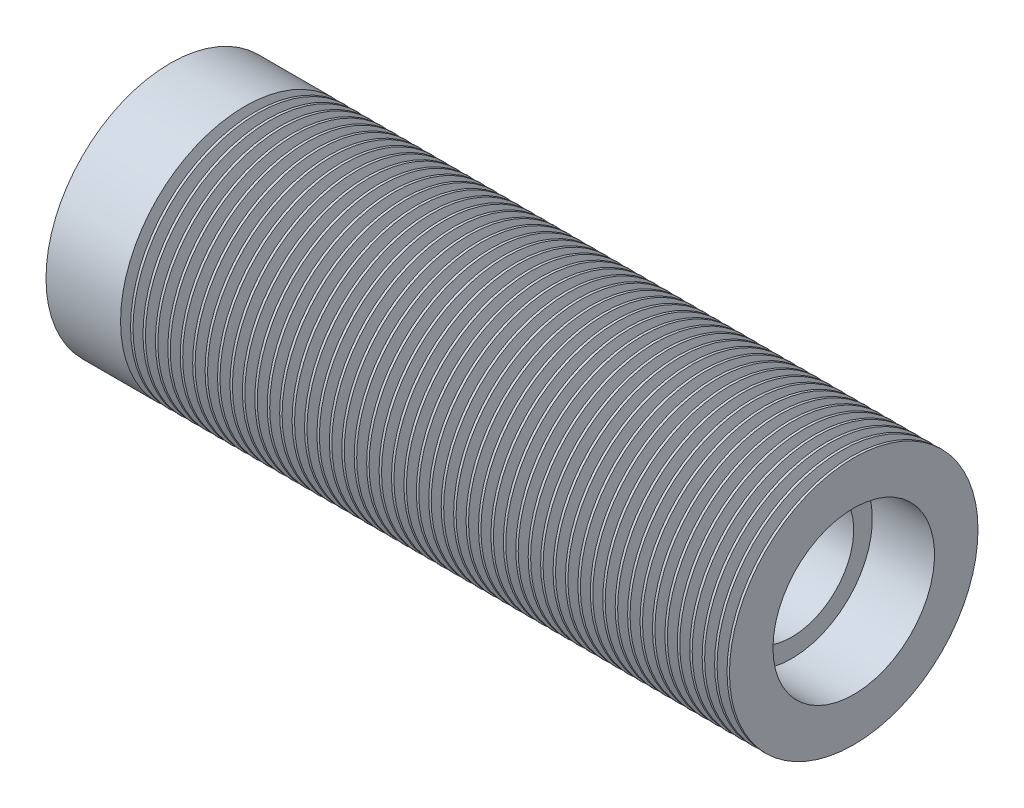
SolidWorks part; units mm, degrees
material "白色铁氟龙"
ref_plane "Front Plane" through (0, 0, 0) normal (0, 0, 1) x (1, 0, 0)
ref_plane "Top Plane" through (0, 0, 0) normal (0, 1, 0) x (1, 0, 0)
ref_plane "Right Plane" through (0, 0, 0) normal (1, 0, 0) x (0, 0, -1)
sketch "Sketch1" plane through (0, 0, 0) normal (0, 0, 1) x (1, 0, 0)
  line L0 (0, 0) -> (49.6022, 0) construction
  line L1 (0, 6.5) -> (0, 10)
  line L2 (0, 10) -> (6, 10)
  line L3 (55, 10) -> (55, 6.5)
  line L4 (55, 6.5) -> (50, 6.5)
  line L5 (50, 6.5) -> (50, 5)
  line L6 (50, 5) -> (5, 5)
  line L7 (5, 5) -> (5, 6.5)
  line L8 (5, 6.5) -> (0, 6.5)
  line L9 (6, 10) -> (6.4019, 8.5)
  line L10 (6.4019, 8.5) -> (6.8038, 10)
  line L11 (6.4019, 10) -> (6.4019, 8.5) construction
  line L12 (7, 10) -> (7.4019, 8.5)
  line L13 (7.4019, 8.5) -> (7.8038, 10)
  line L14 (7.4019, 10) -> (7.4019, 8.5) construction
  line L15 (8, 10) -> (8.4019, 8.5)
  line L16 (8.4019, 8.5) -> (8.8038, 10)
  line L17 (8.4019, 10) -> (8.4019, 8.5) construction
  line L18 (9, 10) -> (9.4019, 8.5)
  line L19 (9.4019, 8.5) -> (9.8038, 10)
  line L20 (9.4019, 10) -> (9.4019, 8.5) construction
  line L21 (10, 10) -> (10.4019, 8.5)
  line L22 (10.4019, 8.5) -> (10.8038, 10)
  line L23 (10.4019, 10) -> (10.4019, 8.5) construction
  line L24 (11, 10) -> (11.4019, 8.5)
  line L25 (11.4019, 8.5) -> (11.8038, 10)
  line L26 (11.4019, 10) -> (11.4019, 8.5) construction
  line L27 (12, 10) -> (12.4019, 8.5)
  line L28 (12.4019, 8.5) -> (12.8038, 10)
  line L29 (12.4019, 10) -> (12.4019, 8.5) construction
  line L30 (13, 10) -> (13.4019, 8.5)
  line L31 (13.4019, 8.5) -> (13.8038, 10)
  line L32 (13.4019, 10) -> (13.4019, 8.5) construction
  line L33 (14, 10) -> (14.4019, 8.5)
  line L34 (14.4019, 8.5) -> (14.8038, 10)
  line L35 (14.4019, 10) -> (14.4019, 8.5) construction
  line L36 (15, 10) -> (15.4019, 8.5)
  line L37 (15.4019, 8.5) -> (15.8038, 10)
  line L38 (15.4019, 10) -> (15.4019, 8.5) construction
  line L39 (16, 10) -> (16.4019, 8.5)
  line L40 (16.4019, 8.5) -> (16.8038, 10)
  line L41 (16.4019, 10) -> (16.4019, 8.5) construction
  line L42 (17, 10) -> (17.4019, 8.5)
  line L43 (17.4019, 8.5) -> (17.8038, 10)
  line L44 (17.4019, 10) -> (17.4019, 8.5) construction
  line L45 (18, 10) -> (18.4019, 8.5)
  line L46 (18.4019, 8.5) -> (18.8038, 10)
  line L47 (18.4019, 10) -> (18.4019, 8.5) construction
  line L48 (19, 10) -> (19.4019, 8.5)
  line L49 (19.4019, 8.5) -> (19.8038, 10)
  line L50 (19.4019, 10) -> (19.4019, 8.5) construction
  line L51 (20, 10) -> (20.4019, 8.5)
  line L52 (20.4019, 8.5) -> (20.8038, 10)
  line L53 (20.4019, 10) -> (20.4019, 8.5) construction
  line L54 (21, 10) -> (21.4019, 8.5)
  line L55 (21.4019, 8.5) -> (21.8038, 10)
  line L56 (21.4019, 10) -> (21.4019, 8.5) construction
  line L57 (22, 10) -> (22.4019, 8.5)
  line L58 (22.4019, 8.5) -> (22.8038, 10)
  line L59 (22.4019, 10) -> (22.4019, 8.5) construction
  line L60 (23, 10) -> (23.4019, 8.5)
  line L61 (23.4019, 8.5) -> (23.8038, 10)
  line L62 (23.4019, 10) -> (23.4019, 8.5) construction
  line L63 (24, 10) -> (24.4019, 8.5)
  line L64 (24.4019, 8.5) -> (24.8038, 10)
  line L65 (24.4019, 10) -> (24.4019, 8.5) construction
  line L66 (25, 10) -> (25.4019, 8.5)
  line L67 (25.4019, 8.5) -> (25.8038, 10)
  line L68 (25.4019, 10) -> (25.4019, 8.5) construction
  line L69 (26, 10) -> (26.4019, 8.5)
  line L70 (26.4019, 8.5) -> (26.8038, 10)
  line L71 (26.4019, 10) -> (26.4019, 8.5) construction
  line L72 (27, 10) -> (27.4019, 8.5)
  line L73 (27.4019, 8.5) -> (27.8038, 10)
  line L74 (27.4019, 10) -> (27.4019, 8.5) construction
  line L75 (28, 10) -> (28.4019, 8.5)
  line L76 (28.4019, 8.5) -> (28.8038, 10)
  line L77 (28.4019, 10) -> (28.4019, 8.5) construction
  line L78 (29, 10) -> (29.4019, 8.5)
  line L79 (29.4019, 8.5) -> (29.8038, 10)
  line L80 (29.4019, 10) -> (29.4019, 8.5) construction
  line L81 (30, 10) -> (30.4019, 8.5)
  line L82 (30.4019, 8.5) -> (30.8038, 10)
  line L83 (30.4019, 10) -> (30.4019, 8.5) construction
  line L84 (31, 10) -> (31.4019, 8.5)
  line L85 (31.4019, 8.5) -> (31.8038, 10)
  line L86 (31.4019, 10) -> (31.4019, 8.5) construction
  line L87 (32, 10) -> (32.4019, 8.5)
  line L88 (32.4019, 8.5) -> (32.8038, 10)
  line L89 (32.4019, 10) -> (32.4019, 8.5) construction
  line L90 (33, 10) -> (33.4019, 8.5)
  line L91 (33.4019, 8.5) -> (33.8038, 10)
  line L92 (33.4019, 10) -> (33.4019, 8.5) construction
  line L93 (34, 10) -> (34.4019, 8.5)
  line L94 (34.4019, 8.5) -> (34.8038, 10)
  line L95 (34.4019, 10) -> (34.4019, 8.5) construction
  line L96 (35, 10) -> (35.4019, 8.5)
  line L97 (35.4019, 8.5) -> (35.8038, 10)
  line L98 (35.4019, 10) -> (35.4019, 8.5) construction
  line L99 (36, 10) -> (36.4019, 8.5)
  line L100 (36.4019, 8.5) -> (36.8038, 10)
  line L101 (36.4019, 10) -> (36.4019, 8.5) construction
  line L102 (37, 10) -> (37.4019, 8.5)
  line L103 (37.4019, 8.5) -> (37.8038, 10)
  line L104 (37.4019, 10) -> (37.4019, 8.5) construction
  line L105 (38, 10) -> (38.4019, 8.5)
  line L106 (38.4019, 8.5) -> (38.8038, 10)
  line L107 (38.4019, 10) -> (38.4019, 8.5) construction
  line L108 (39, 10) -> (39.4019, 8.5)
  line L109 (39.4019, 8.5) -> (39.8038, 10)
  line L110 (39.4019, 10) -> (39.4019, 8.5) construction
  line L111 (40, 10) -> (40.4019, 8.5)
  line L112 (40.4019, 8.5) -> (40.8038, 10)
  line L113 (40.4019, 10) -> (40.4019, 8.5) construction
  line L114 (41, 10) -> (41.4019, 8.5)
  line L115 (41.4019, 8.5) -> (41.8038, 10)
  line L116 (41.4019, 10) -> (41.4019, 8.5) construction
  line L117 (42, 10) -> (42.4019, 8.5)
  line L118 (42.4019, 8.5) -> (42.8038, 10)
  line L119 (42.4019, 10) -> (42.4019, 8.5) construction
  line L120 (43, 10) -> (43.4019, 8.5)
  line L121 (43.4019, 8.5) -> (43.8038, 10)
  line L122 (43.4019, 10) -> (43.4019, 8.5) construction
  line L123 (44, 10) -> (44.4019, 8.5)
  line L124 (44.4019, 8.5) -> (44.8038, 10)
  line L125 (44.4019, 10) -> (44.4019, 8.5) construction
  line L126 (45, 10) -> (45.4019, 8.5)
  line L127 (45.4019, 8.5) -> (45.8038, 10)
  line L128 (45.4019, 10) -> (45.4019, 8.5) construction
  line L129 (46, 10) -> (46.4019, 8.5)
  line L130 (46.4019, 8.5) -> (46.8038, 10)
  line L131 (46.4019, 10) -> (46.4019, 8.5) construction
  line L132 (47, 10) -> (47.4019, 8.5)
  line L133 (47.4019, 8.5) -> (47.8038, 10)
  line L134 (47.4019, 10) -> (47.4019, 8.5) construction
  line L135 (6.8038, 10) -> (7, 10)
  line L136 (7.8038, 10) -> (8, 10)
  line L137 (8.8038, 10) -> (9, 10)
  line L138 (9.8038, 10) -> (10, 10)
  line L139 (10.8038, 10) -> (11, 10)
  line L140 (11.8038, 10) -> (12, 10)
  line L141 (12.8038, 10) -> (13, 10)
  line L142 (13.8038, 10) -> (14, 10)
  line L143 (14.8038, 10) -> (15, 10)
  line L144 (15.8038, 10) -> (16, 10)
  line L145 (16.8038, 10) -> (17, 10)
  line L146 (17.8038, 10) -> (18, 10)
  line L147 (18.8038, 10) -> (19, 10)
  line L148 (19.8038, 10) -> (20, 10)
  line L149 (20.8038, 10) -> (21, 10)
  line L150 (21.8038, 10) -> (22, 10)
  line L151 (22.8038, 10) -> (23, 10)
  line L152 (23.8038, 10) -> (24, 10)
  line L153 (24.8038, 10) -> (25, 10)
  line L154 (25.8038, 10) -> (26, 10)
  line L155 (26.8038, 10) -> (27, 10)
  line L156 (27.8038, 10) -> (28, 10)
  line L157 (28.8038, 10) -> (29, 10)
  line L158 (29.8038, 10) -> (30, 10)
  line L159 (30.8038, 10) -> (31, 10)
  line L160 (31.8038, 10) -> (32, 10)
  line L161 (32.8038, 10) -> (33, 10)
  line L162 (33.8038, 10) -> (34, 10)
  line L163 (34.8038, 10) -> (35, 10)
  line L164 (35.8038, 10) -> (36, 10)
  line L165 (36.8038, 10) -> (37, 10)
  line L166 (37.8038, 10) -> (38, 10)
  line L167 (38.8038, 10) -> (39, 10)
  line L168 (39.8038, 10) -> (40, 10)
  line L169 (40.8038, 10) -> (41, 10)
  line L170 (41.8038, 10) -> (42, 10)
  line L171 (42.8038, 10) -> (43, 10)
  line L172 (43.8038, 10) -> (44, 10)
  line L173 (44.8038, 10) -> (45, 10)
  line L174 (45.8038, 10) -> (46, 10)
  line L175 (46.8038, 10) -> (47, 10)
  line L176 (47.8038, 10) -> (48, 10)
  line L177 (48, 10) -> (48.4019, 8.5)
  line L178 (48.4019, 8.5) -> (48.8038, 10)
  line L179 (49, 10) -> (49.4019, 8.5)
  line L180 (49.4019, 8.5) -> (49.8038, 10)
  line L181 (50, 10) -> (50.4019, 8.5)
  line L182 (50.4019, 8.5) -> (50.8038, 10)
  line L183 (51, 10) -> (51.4019, 8.5)
  line L184 (51.4019, 8.5) -> (51.8038, 10)
  line L185 (52, 10) -> (52.4019, 8.5)
  line L186 (52.4019, 8.5) -> (52.8038, 10)
  line L187 (53, 10) -> (53.4019, 8.5)
  line L188 (53.4019, 8.5) -> (53.8038, 10)
  line L189 (54, 10) -> (54.4019, 8.5)
  line L190 (54.4019, 8.5) -> (54.8038, 10)
  line L191 (48.8038, 10) -> (49, 10)
  line L192 (49.8038, 10) -> (50, 10)
  line L193 (50.8038, 10) -> (51, 10)
  line L194 (51.8038, 10) -> (52, 10)
  line L195 (52.8038, 10) -> (53, 10)
  line L196 (53.8038, 10) -> (54, 10)
  line L197 (54.8038, 10) -> (55, 10)
  dimension "D1" = 6.5
  dimension "D2" = 10
  dimension "D3" = 5
  dimension "D4" = 5
  dimension "D5" = 5
  dimension "D6" = 55
  dimension "D7" = 1.5
  dimension "D8" = 30
  dimension "D9" = 6
  dimension "D11" = 1
  dimension "D12" = 8
  dimension "D13" = 1
  dimension "D10" = 42
revolve "Revolve1" add sketch "Sketch1" angle 360 about L0
